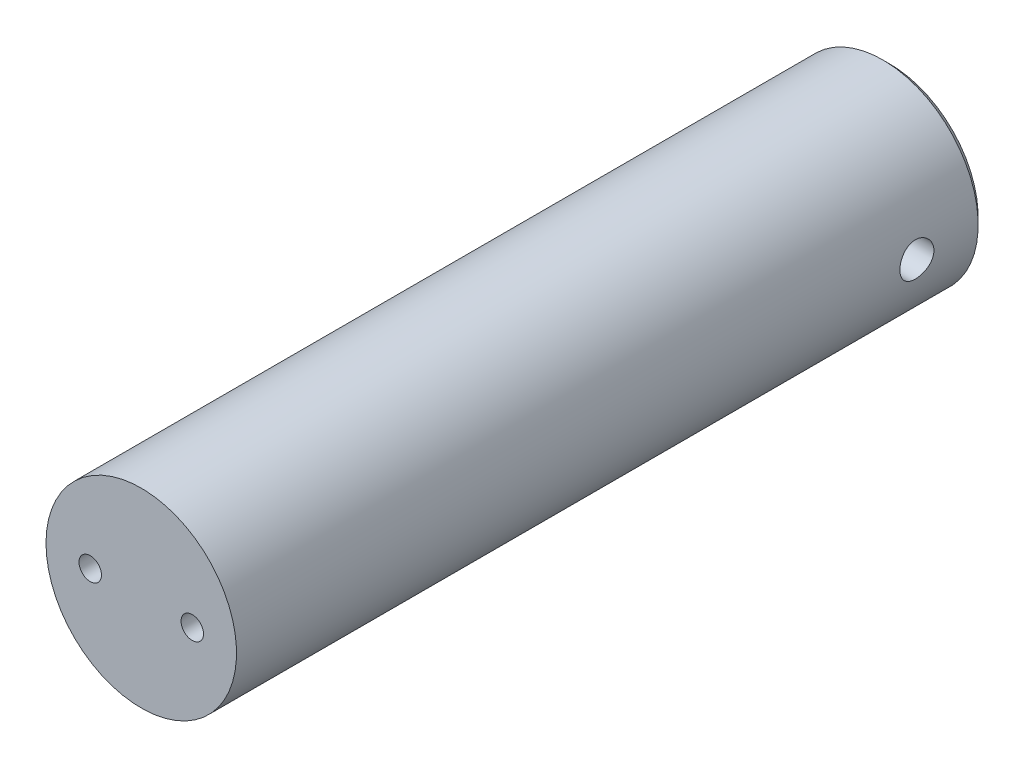
from build123d import *

# Parameters (mm, degrees)
M4_TAPPED_HOLE1_D     = 3.3
M4_TAPPED_HOLE1_DEPTH = 10.1
M4_TAPPED_HOLE1_TIP   = 0.991420021
M6_TAPPED_HOLE1_D     = 5
M6_TAPPED_HOLE1_DEPTH = 17
M6_TAPPED_HOLE1_TIP   = 1.502151548
CHAMFER1_SIZE         = 1


with BuildPart() as part:
    # Sketch1 → Revolve1 (revolve)
    with BuildSketch(Plane(origin=(0, 0, 0), x_dir=(1, 0, 0), z_dir=(0, 1, 0))):
        Polygon((-9.05, 110), (-14, 110), (-14, 0), (0, 0), (0, 50), (-9.05, 50), align=None)
    revolve(axis=Axis((0, 0, -50), (0, 0, 1)))

    # M4 Tapped Hole1
    with Locations(Plane(origin=(-7.5, 0, 0), x_dir=(1, 0, 0), z_dir=(0, 0, 1))):
        with Locations((0, 0), (15, 0)):
            Hole(M4_TAPPED_HOLE1_D / 2, depth=M4_TAPPED_HOLE1_DEPTH)
            with Locations((0, 0, -(M4_TAPPED_HOLE1_DEPTH + M4_TAPPED_HOLE1_TIP / 2))):  # 118° drill point
                Cone(0, M4_TAPPED_HOLE1_D / 2, M4_TAPPED_HOLE1_TIP, mode=Mode.SUBTRACT)

    # M6 Tapped Hole1
    with Locations(Plane(origin=(14, 0, -100), x_dir=(0, 1, 0), z_dir=(1, 0, 0))):
        with Locations((0, 0)):
            Hole(M6_TAPPED_HOLE1_D / 2, depth=M6_TAPPED_HOLE1_DEPTH)
            with Locations((0, 0, -(M6_TAPPED_HOLE1_DEPTH + M6_TAPPED_HOLE1_TIP / 2))):  # 118° drill point
                Cone(0, M6_TAPPED_HOLE1_D / 2, M6_TAPPED_HOLE1_TIP, mode=Mode.SUBTRACT)

    # Chamfer1
    chamfer1_edges = [part.edges().sort_by_distance(p)[0] for p in [
        (14, 0, -110),
        (9.05, 0, -110),
    ]]
    chamfer(chamfer1_edges, length=CHAMFER1_SIZE)


solid = part.part
